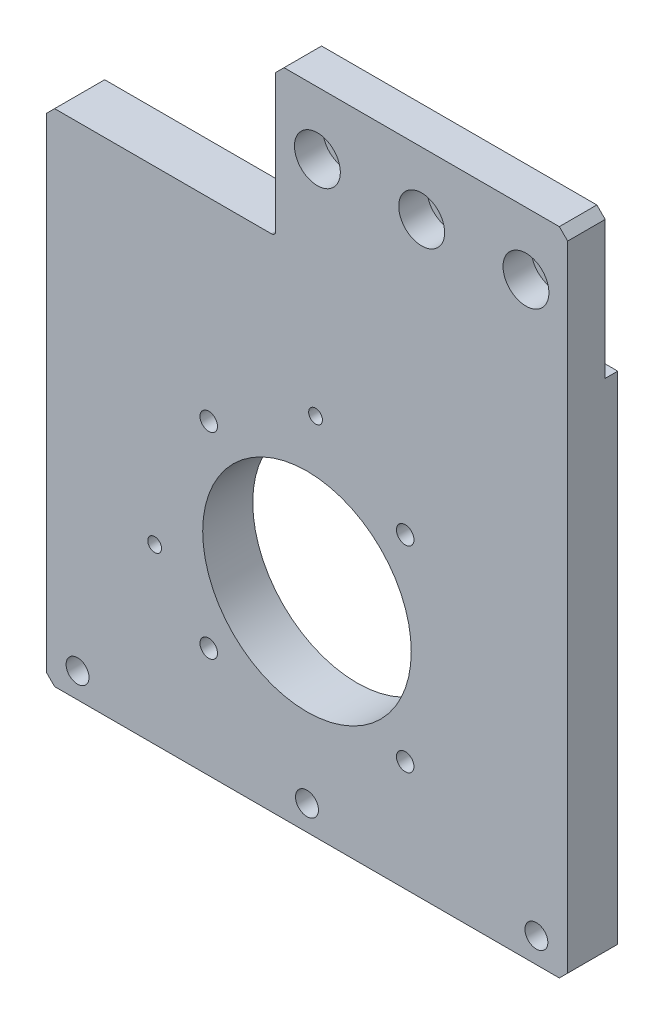
from build123d import *

# Parameters (mm, degrees)
SKETCH_1_W                = 125
SKETCH_1_H                = 156
EXTRUDE_1_DEPTH           = 12
SKETCH_2_W                = 55
SKETCH_2_H                = 36
CUT_EXTRUDE_1_DEPTH       = 101.669012114
SKETCH_3_W                = 70
SKETCH_3_H                = 35
CUT_EXTRUDE_2_DEPTH       = 3
HOLE_WIZARD_1_D           = 5.5
HOLE_WIZARD_1_CBORE_D     = 10
HOLE_WIZARD_1_CBORE_DEPTH = 5.7
HOLE_WIZARD_2_D           = 6.6
HOLE_WIZARD_2_CBORE_D     = 11
HOLE_WIZARD_2_CBORE_DEPTH = 6.8
CHAMFER_1_SIZE            = 2
FILLET_1_R                = 1
SKETCH_10_R               = 25
CUT_EXTRUDE_3_DEPTH       = 101.669012114
HOLE_WIZARD_M5_1_D        = 4.2
HOLE_WIZARD_M4_1_D        = 3.3


with BuildPart() as part:
    # 草图1 → 凸台-拉伸1 (new body)
    with BuildSketch(Plane.XY):
        Rectangle(SKETCH_1_W, SKETCH_1_H)
    extrude(amount=EXTRUDE_1_DEPTH)

    # 草图2 → 切除-拉伸1 (cut, through all)
    with BuildSketch(Plane.XY.offset(12)):
        with Locations((-35, 60)):
            Rectangle(SKETCH_2_W, SKETCH_2_H)
    extrude(amount=-CUT_EXTRUDE_1_DEPTH, mode=Mode.SUBTRACT)

    # 草图3 → 切除-拉伸2 (cut)
    with BuildSketch(Plane(origin=(0, 0, 0), x_dir=(-1, 0, 0), z_dir=(0, 0, -1))):
        with Locations((-27.5, 60.5)):
            Rectangle(SKETCH_3_W, SKETCH_3_H)
    extrude(amount=-CUT_EXTRUDE_2_DEPTH, mode=Mode.SUBTRACT)

    # 打孔尺寸(%根据)内六角圆柱头螺钉的类型1 (through all)
    with Locations(Plane(origin=(0, 0, 0), x_dir=(-1, 0, 0), z_dir=(0, 0, -1))):
        with Locations((-55, -72), (0, -72), (55, -72)):
            CounterBoreHole(HOLE_WIZARD_1_D / 2, HOLE_WIZARD_1_CBORE_D / 2, HOLE_WIZARD_1_CBORE_DEPTH)

    # 打孔尺寸(%根据)内六角圆柱头螺钉的类型2 (through all)
    with Locations(Plane(origin=(0, 0, 12), x_dir=(-1, 0, 0), z_dir=(0, 0, 1))):
        with Locations((-52.5, -63), (-27.5, -63), (-2.5, -63)):
            CounterBoreHole(HOLE_WIZARD_2_D / 2, HOLE_WIZARD_2_CBORE_D / 2, HOLE_WIZARD_2_CBORE_DEPTH)

    # 倒角1
    chamfer_1_edges = [part.edges().sort_by_distance(p)[0] for p in [
        (-62.5, 42, 6),
        (-7.5, 78, 7.5),
        (62.5, -78, 6),
        (-62.5, -78, 6),
        (62.5, 78, 7.5),
    ]]
    chamfer(chamfer_1_edges, length=CHAMFER_1_SIZE)

    # 圆角1
    fillet_1_edges = [part.edges().sort_by_distance(p)[0] for p in [
        (-7.5, 42, 6),
    ]]
    fillet(fillet_1_edges, radius=FILLET_1_R)

    # 草图10 → 切除-拉伸3 (cut, through all)
    with BuildSketch(Plane.XY.offset(12)):
        with Locations((0, -28)):
            Circle(SKETCH_10_R)
    extrude(amount=-CUT_EXTRUDE_3_DEPTH, mode=Mode.SUBTRACT)

    # M5 螺纹孔1 (through all)
    with Locations(Plane(origin=(0, 0, 0), x_dir=(-1, 0, 0), z_dir=(0, 0, -1))):
        with Locations((-23.55, -4.45), (23.55, -4.45), (23.55, -51.55), (-23.55, -51.55)):
            Hole(HOLE_WIZARD_M5_1_D / 2)

    # M4 螺纹孔1 (through all)
    with Locations(Plane.XY.offset(12)):
        with Locations((2.053366632, 9.443740271), (-36.520933317, -36.513015309)):
            Hole(HOLE_WIZARD_M4_1_D / 2)


solid = part.part
